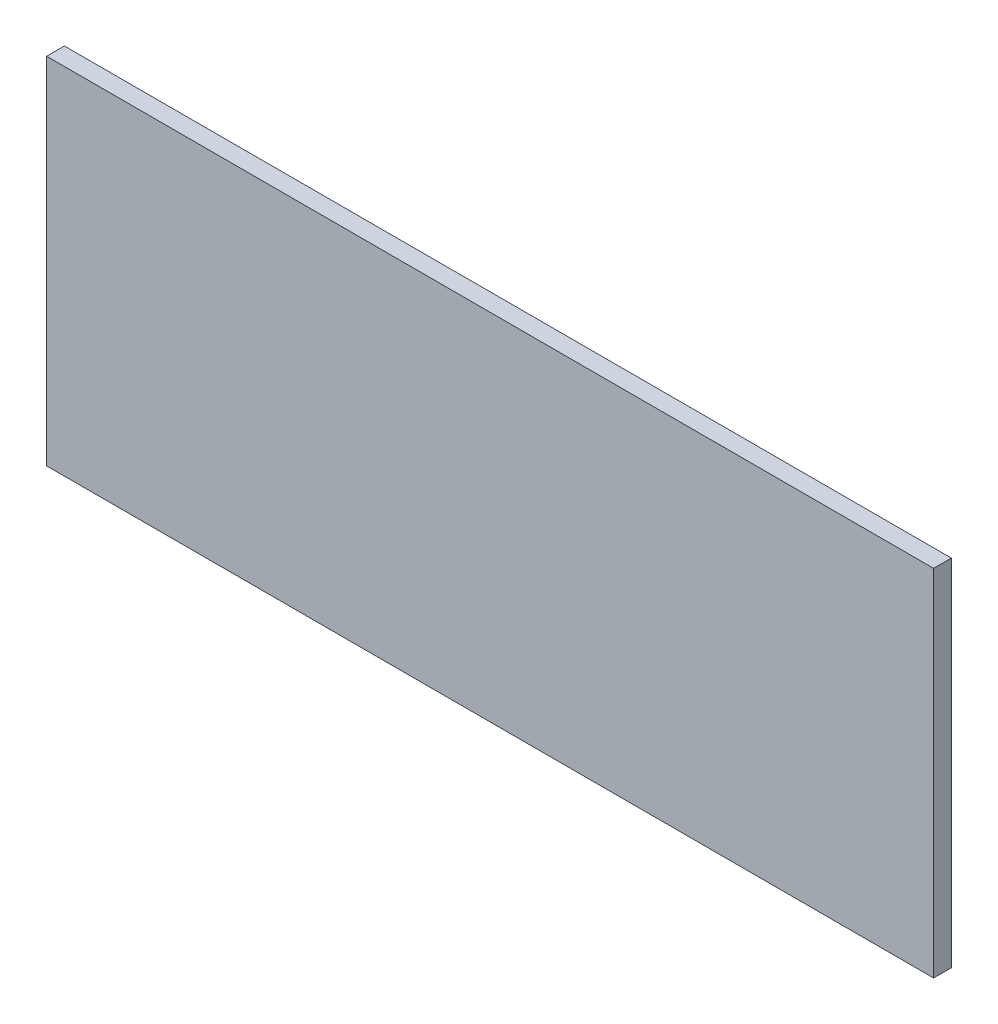
from build123d import *

# Parameters (mm, degrees)
SKETCH1_W           = 5000
SKETCH1_H           = 2000
BOSS_EXTRUDE1_DEPTH = 100


with BuildPart() as part:
    # Sketch1 → Boss-Extrude1 (new body)
    with BuildSketch(Plane.XY):
        with Locations((2500, 1000)):
            Rectangle(SKETCH1_W, SKETCH1_H)
    extrude(amount=BOSS_EXTRUDE1_DEPTH)


solid = part.part
